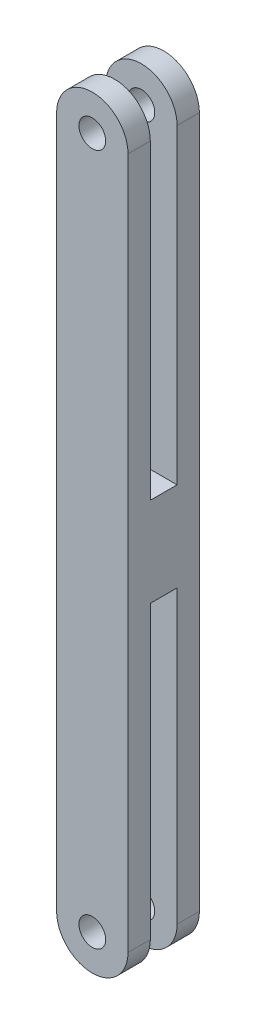
from build123d import *

# Parameters (mm, degrees)
SKETCH1_R           = 3
BOSS_EXTRUDE1_DEPTH = 16
SKETCH2_W           = 6
SKETCH2_H           = 139.453359721
SKETCH2_H_2         = 146.546640279
CUT_EXTRUDE1_DEPTH  = 91.59784964


with BuildPart() as part:
    # Sketch1 → Boss-Extrude1 (new body)
    with BuildSketch(Plane.XY):
        with BuildLine():
            Line((-8, 79.726679861), (-8, -75.273320139))
            ThreePointArc((-8, -75.273320139), (0, -83.273320139), (8, -75.273320139))
            Line((8, -75.273320139), (8, 79.726679861))
            ThreePointArc((8, 79.726679861), (0, 87.726679861), (-8, 79.726679861))
        make_face()
        with Locations((0, 79.726679861)):
            Circle(SKETCH1_R, mode=Mode.SUBTRACT)
        with Locations((0, -75.273320139)):
            Circle(SKETCH1_R, mode=Mode.SUBTRACT)
    extrude(amount=BOSS_EXTRUDE1_DEPTH)

    # Sketch2 → Cut-Extrude1 (cut, through all)
    with BuildSketch(Plane(origin=(8, 0, 0), x_dir=(0, 0, -1), z_dir=(1, 0, 0))):
        with Locations((-8, 79.72667986)):
            Rectangle(SKETCH2_W, SKETCH2_H)
        with Locations((-8, -83.27332014)):
            Rectangle(SKETCH2_W, SKETCH2_H_2)
    extrude(amount=-CUT_EXTRUDE1_DEPTH, mode=Mode.SUBTRACT)


solid = part.part
